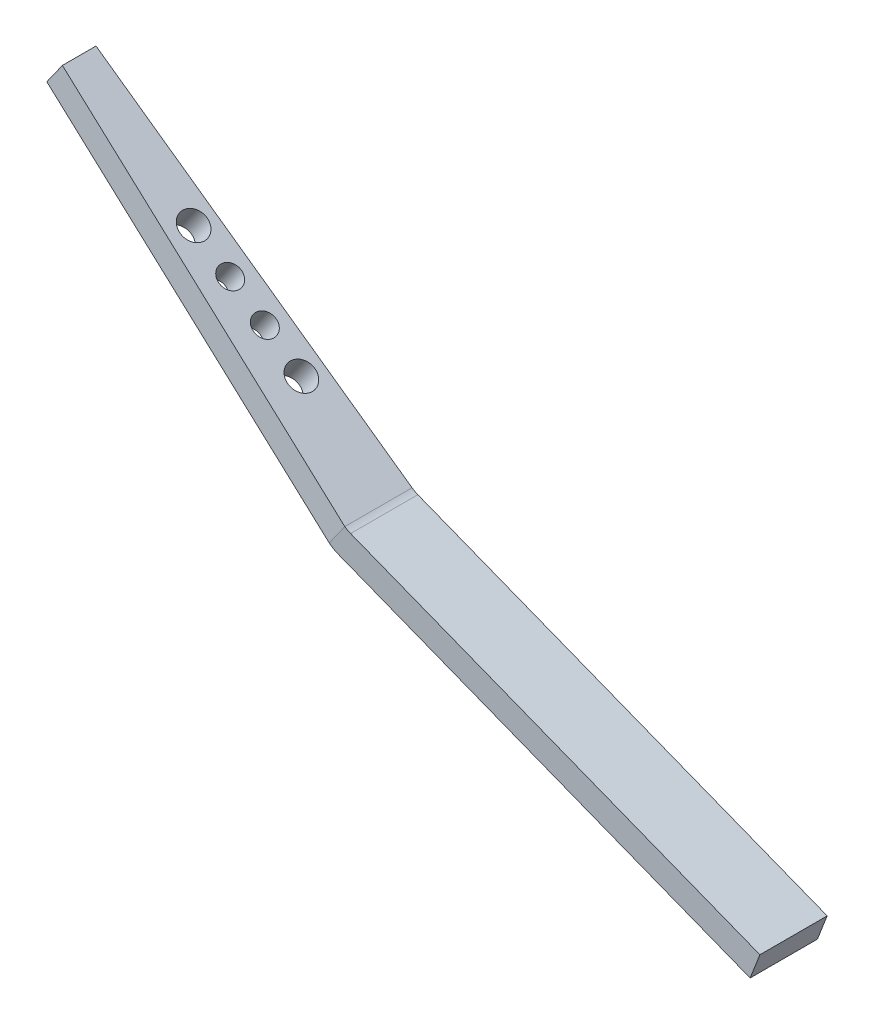
from build123d import *

# Parameters (mm, degrees)
EXTRUDE_1_DEPTH     = 15
CUT_EXTRUDE_1_DEPTH = 20
MM_1_D              = 6
HOLE_WIZARD_M6_1_D  = 5


with BuildPart() as part:
    # 草图1 → 凸台-拉伸1 (new body)
    with BuildSketch(Plane.XY):
        with BuildLine():
            Line((-145.547396155, 197.773537563), (-142.072104357, 202.664585193))
            Line((-142.072104357, 202.664585193), (-71.595844229, 152.588285115))
            ThreePointArc((-71.595844229, 152.588285115), (-70.97220164, 152.200308518), (-70.305827411, 151.891437501))
            Line((-70.305827411, 151.891437501), (20.980591756, 116.19178332))
            Line((20.980591756, 116.19178332), (18.795316776, 110.603888076))
            Line((18.795316776, 110.603888076), (-73.179003731, 146.5725619))
            ThreePointArc((-73.179003731, 146.5725619), (-73.84537796, 146.881432918), (-74.469020549, 147.269409515))
            Line((-74.469020549, 147.269409515), (-145.547396155, 197.773537563))
        make_face()
    extrude(amount=EXTRUDE_1_DEPTH)

    # 草图3 → 切除-拉伸1 (cut)
    with BuildSketch(Plane(origin=(48.026613519, 67.591577297, 0), x_dir=(0.8151746049568696, -0.5792152997231786, 0), z_dir=(0.5792152997231786, 0.8151746049568696, 0))):
        Polygon((-233.2, -7.5), (-146.744583334, -15), (-233.2, -15), align=None)
    extrude(amount=-CUT_EXTRUDE_1_DEPTH, mode=Mode.SUBTRACT)

    # 大小mm 暗销孔1 (through all)
    with Locations(Plane(origin=(48.026613519, 67.591577297, 0), x_dir=(0.8151746049568697, -0.5792152997231785, 0), z_dir=(0.5792152997231785, 0.8151746049568697, 0))):
        with Locations((-200.523492287, -4.870838518), (-171.040138216, -4.870838518)):
            Hole(MM_1_D / 2)

    # M6 螺纹孔1 (through all)
    with Locations(Plane(origin=(48.026613519, 67.591577297, 0), x_dir=(0.8151746049568697, -0.5792152997231785, 0), z_dir=(0.5792152997231785, 0.8151746049568697, 0))):
        with Locations((-190.523492287, -4.870838518), (-181.040138216, -4.870838518)):
            Hole(HOLE_WIZARD_M6_1_D / 2)


solid = part.part
